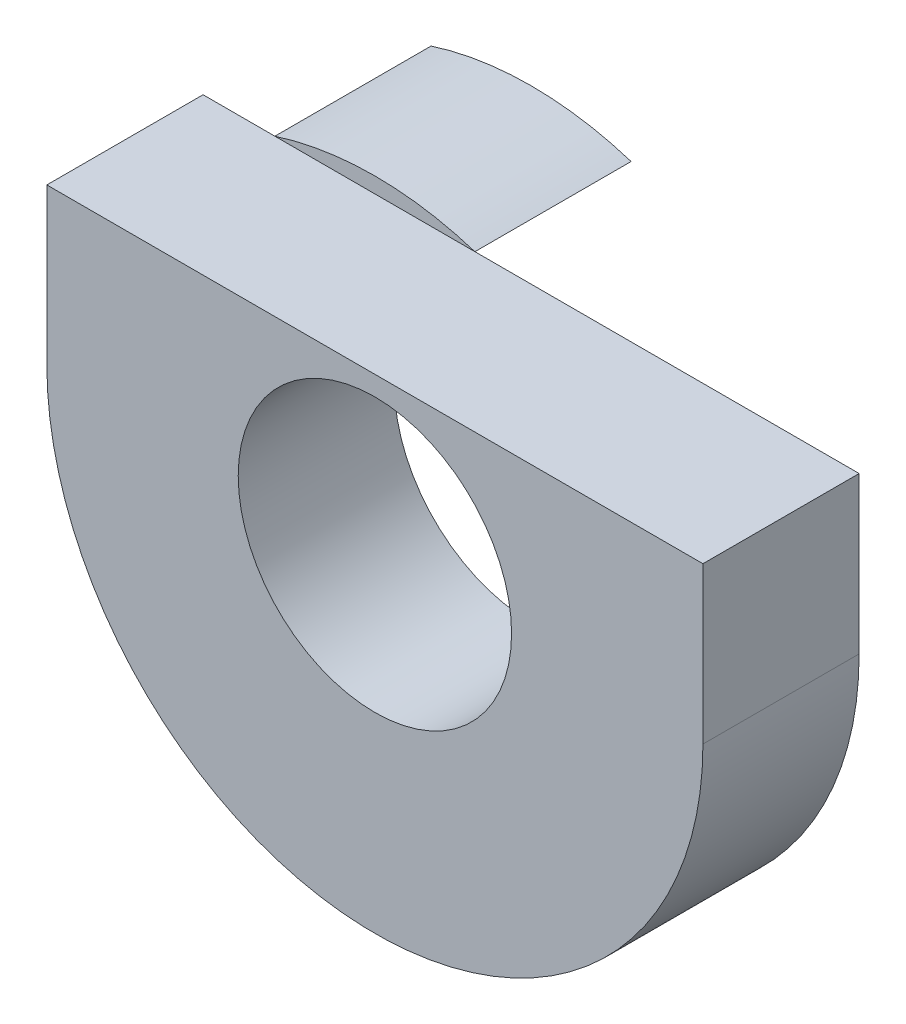
SolidWorks part; units mm, degrees
ref_plane "Front Plane" through (0, 0, 0) normal (0, 0, 1) x (1, 0, 0)
ref_plane "Top Plane" through (0, 0, 0) normal (0, 1, 0) x (1, 0, 0)
ref_plane "Right Plane" through (0, 0, 0) normal (1, 0, 0) x (0, 0, -1)
other "Configuration Table"
sketch "Sketch1" plane through (0, 0, 0) normal (0, 0, 1) x (1, 0, 0)
  circle A0 centre (0, 0) radius 210
  circle A1 centre (0, 0) radius 87.5
  dimension "D1" = 175
  dimension "D2" = 420
extrude "Boss-Extrude1" add sketch "Sketch1" along normal blind 100
sketch "Sketch2" plane through (0, 0, 100) normal (0, 0, 1) x (1, 0, 0)
  line L0 (87.5, 0) -> (210, 0)
  line L1 (-210, 0) -> (-87.5, 0)
  line L2 (-210, 0) -> (-210, 100)
  line L3 (-210, 100) -> (210, 100)
  line L4 (210, 0) -> (210, 100)
  circle A0 centre (0, 0) radius 210 construction
  circle A1 centre (0, 0) radius 87.5 construction
  arc A2 (87.5, 0) -> (-87.5, 0) centre (0, 0) ccw
  dimension "D1" = 100
extrude "Boss-Extrude2" add sketch "Sketch2" against normal up to surface (100 mm away) up to face at (210, 0, 0)
sketch "Sketch3" plane through (0, 0, 0) normal (0, 0, -1) x (-1, 0, 0)
  line L1 (-184.6619, 100) -> (184.6619, 100)
  line L2 (-184.6619, 100) -> (-184.6619, 200)
  line L3 (-184.6619, 200) -> (184.6619, 200)
  line L4 (184.6619, 100) -> (184.6619, 200)
  dimension "D1" = 100
extrude "Cut-Extrude1" cut sketch "Sketch3" against normal through all
